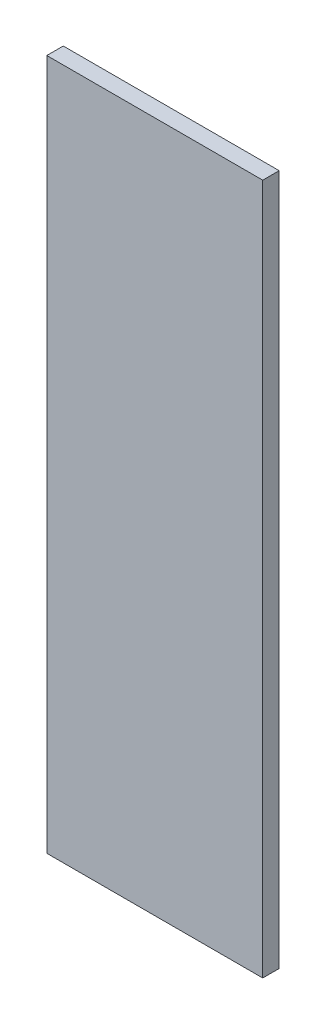
from build123d import *

# Parameters (mm, degrees)
SKETCH1_W           = 105
SKETCH1_H           = 336
BOSS_EXTRUDE1_DEPTH = 4


with BuildPart() as part:
    # Sketch1 → Boss-Extrude1 (new, symmetric)
    with BuildSketch(Plane.XY):
        Rectangle(SKETCH1_W, SKETCH1_H)
    extrude(amount=BOSS_EXTRUDE1_DEPTH, both=True)


solid = part.part
